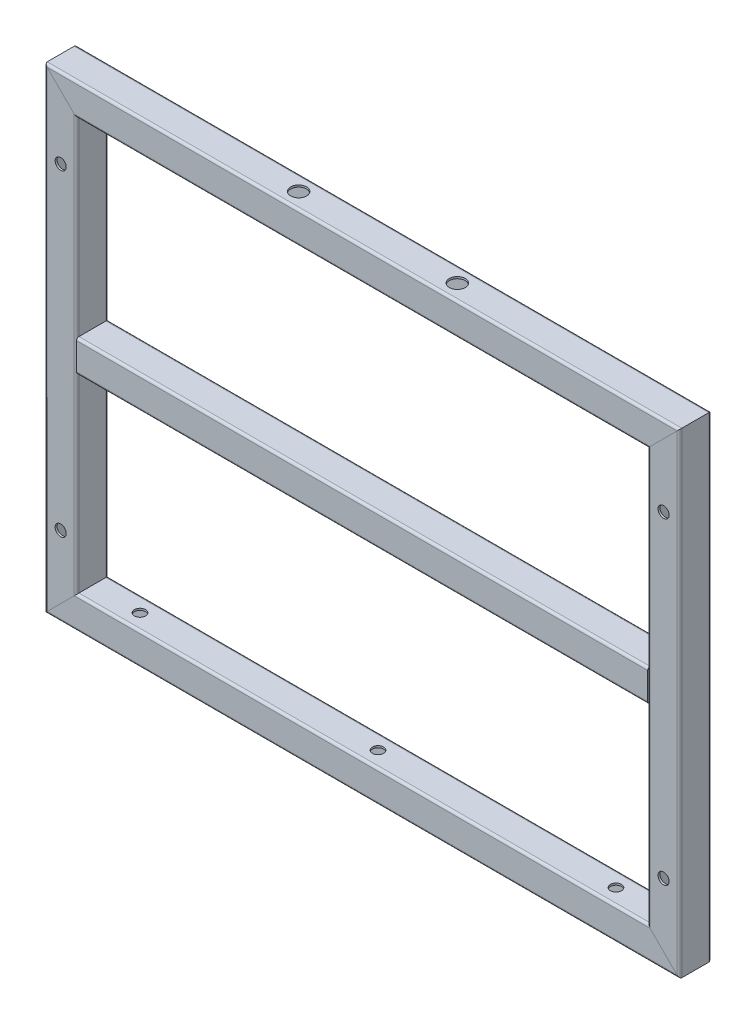
from build123d import *

# Parameters (mm, degrees)
STRUCTURAL_MEMBER1_DEPTH      = 395.142135624
STRUCTURAL_MEMBER1_DEPTH_BACK = 15.142135624
STRUCTURAL_MEMBER1_2_DEPTH    = 310.284271247
STRUCTURAL_MEMBER1_3_DEPTH    = 410.284271247
STRUCTURAL_MEMBER1_4_DEPTH    = 310.284271247
STRUCTURAL_MEMBER1_5_DEPTH    = 382
SKETCH3_R                     = 3.5
CUT_EXTRUDE1_DEPTH            = 251.79872408
SKETCH4_R                     = 5
CUT_EXTRUDE2_DEPTH            = 10
SKETCH5_R                     = 3.5
CUT_EXTRUDE3_DEPTH            = 20


with BuildPart() as part:
    # Sketch1 → Structural Member1 (new, two sides: drawn at the far end of the back side and taken through both)
    with BuildSketch(Plane(origin=(190, 140, 0), x_dir=(0, -1, 0), z_dir=(-1, 0, 0)).offset(-STRUCTURAL_MEMBER1_DEPTH_BACK)):
        with BuildLine():
            Line((-8.5, -10), (8.5, -10))
            ThreePointArc((8.5, -10), (9.560660172, -9.560660172), (10, -8.5))
            Line((10, -8.5), (10, 8.5))
            ThreePointArc((10, 8.5), (9.560660172, 9.560660172), (8.5, 10))
            Line((8.5, 10), (-8.5, 10))
            ThreePointArc((-8.5, 10), (-9.560660172, 9.560660172), (-10, 8.5))
            Line((-10, 8.5), (-10, -8.5))
            ThreePointArc((-10, -8.5), (-9.560660172, -9.560660172), (-8.5, -10))
        make_face()
        with BuildLine():
            Line((-8.5, -8.8), (8.5, -8.8))
            ThreePointArc((8.5, -8.8), (8.712132034, -8.712132034), (8.8, -8.5))
            Line((8.8, -8.5), (8.8, 8.5))
            ThreePointArc((8.8, 8.5), (8.712132034, 8.712132034), (8.5, 8.8))
            Line((8.5, 8.8), (-8.5, 8.8))
            ThreePointArc((-8.5, 8.8), (-8.712132034, 8.712132034), (-8.8, 8.5))
            Line((-8.8, 8.5), (-8.8, -8.5))
            ThreePointArc((-8.8, -8.5), (-8.712132034, -8.712132034), (-8.5, -8.8))
        make_face(mode=Mode.SUBTRACT)
    extrude(amount=STRUCTURAL_MEMBER1_DEPTH + STRUCTURAL_MEMBER1_DEPTH_BACK)

    # Structural Member1 mitre 1
    split(bisect_by=Plane(origin=(190, 140, 0), x_dir=(-0.707106781, -0.707106781, 0), z_dir=(-0.707106781, 0.707106781, 0)), keep=Keep.TOP)

    # Structural Member1 mitre 2
    split(bisect_by=Plane(origin=(-190, 140, 0), x_dir=(-0.707106781, 0.707106781, 0), z_dir=(0.707106781, 0.707106781, 0)), keep=Keep.TOP)

    # Sketch4 → Cut-Extrude2 (cut)
    with BuildSketch(Plane(origin=(0, 150, 0), x_dir=(-1, 0, 0), z_dir=(0, 1, 0))):
        with Locations((50, 0)):
            Circle(SKETCH4_R)
        with Locations((-50, 0)):
            Circle(SKETCH4_R)
    extrude(amount=-CUT_EXTRUDE2_DEPTH, mode=Mode.SUBTRACT)


with BuildPart() as body_2:
    # Sketch1 on segment 2 (carried to segment 2) → Structural Member1 2 (new body)
    with BuildSketch(Plane(origin=(-190, 155.142135624, 0), x_dir=(1, 0, 0), z_dir=(0, -1, 0))):
        with BuildLine():
            Line((-8.5, -10), (8.5, -10))
            ThreePointArc((8.5, -10), (9.560660172, -9.560660172), (10, -8.5))
            Line((10, -8.5), (10, 8.5))
            ThreePointArc((10, 8.5), (9.560660172, 9.560660172), (8.5, 10))
            Line((8.5, 10), (-8.5, 10))
            ThreePointArc((-8.5, 10), (-9.560660172, 9.560660172), (-10, 8.5))
            Line((-10, 8.5), (-10, -8.5))
            ThreePointArc((-10, -8.5), (-9.560660172, -9.560660172), (-8.5, -10))
        make_face()
        with BuildLine():
            Line((-8.5, -8.8), (8.5, -8.8))
            ThreePointArc((8.5, -8.8), (8.712132034, -8.712132034), (8.8, -8.5))
            Line((8.8, -8.5), (8.8, 8.5))
            ThreePointArc((8.8, 8.5), (8.712132034, 8.712132034), (8.5, 8.8))
            Line((8.5, 8.8), (-8.5, 8.8))
            ThreePointArc((-8.5, 8.8), (-8.712132034, 8.712132034), (-8.8, 8.5))
            Line((-8.8, 8.5), (-8.8, -8.5))
            ThreePointArc((-8.8, -8.5), (-8.712132034, -8.712132034), (-8.5, -8.8))
        make_face(mode=Mode.SUBTRACT)
    extrude(amount=STRUCTURAL_MEMBER1_2_DEPTH)

    # Structural Member1 2 mitre 1
    split(bisect_by=Plane(origin=(-190, 140, 0), x_dir=(0.707106781, -0.707106781, 0), z_dir=(-0.707106781, -0.707106781, 0)), keep=Keep.TOP)

    # Structural Member1 2 mitre 2
    split(bisect_by=Plane(origin=(-190, -140, 0), x_dir=(-0.707106781, -0.707106781, 0), z_dir=(-0.707106781, 0.707106781, 0)), keep=Keep.TOP)


with BuildPart() as body_3:
    # Sketch1 on segment 3 (carried to segment 3) → Structural Member1 3 (new body)
    with BuildSketch(Plane(origin=(-205.142135624, -140, 0), x_dir=(0, 1, 0), z_dir=(1, 0, 0))):
        with BuildLine():
            Line((-8.5, -10), (8.5, -10))
            ThreePointArc((8.5, -10), (9.560660172, -9.560660172), (10, -8.5))
            Line((10, -8.5), (10, 8.5))
            ThreePointArc((10, 8.5), (9.560660172, 9.560660172), (8.5, 10))
            Line((8.5, 10), (-8.5, 10))
            ThreePointArc((-8.5, 10), (-9.560660172, 9.560660172), (-10, 8.5))
            Line((-10, 8.5), (-10, -8.5))
            ThreePointArc((-10, -8.5), (-9.560660172, -9.560660172), (-8.5, -10))
        make_face()
        with BuildLine():
            Line((-8.5, -8.8), (8.5, -8.8))
            ThreePointArc((8.5, -8.8), (8.712132034, -8.712132034), (8.8, -8.5))
            Line((8.8, -8.5), (8.8, 8.5))
            ThreePointArc((8.8, 8.5), (8.712132034, 8.712132034), (8.5, 8.8))
            Line((8.5, 8.8), (-8.5, 8.8))
            ThreePointArc((-8.5, 8.8), (-8.712132034, 8.712132034), (-8.8, 8.5))
            Line((-8.8, 8.5), (-8.8, -8.5))
            ThreePointArc((-8.8, -8.5), (-8.712132034, -8.712132034), (-8.5, -8.8))
        make_face(mode=Mode.SUBTRACT)
    extrude(amount=STRUCTURAL_MEMBER1_3_DEPTH)

    # Structural Member1 3 mitre 1
    split(bisect_by=Plane(origin=(190, -140, 0), x_dir=(0.707106781, -0.707106781, 0), z_dir=(-0.707106781, -0.707106781, 0)), keep=Keep.TOP)

    # Structural Member1 3 mitre 2
    split(bisect_by=Plane(origin=(-190, -140, 0), x_dir=(0.707106781, 0.707106781, 0), z_dir=(0.707106781, -0.707106781, 0)), keep=Keep.TOP)

    # Sketch5 → Cut-Extrude3 (cut)
    with BuildSketch(Plane(origin=(0, -130, 0), x_dir=(-1, 0, 0), z_dir=(0, 1, 0))):
        Circle(SKETCH5_R)
        with Locations((-150, 0)):
            Circle(SKETCH5_R)
        with Locations((150, 0)):
            Circle(SKETCH5_R)
    extrude(amount=-CUT_EXTRUDE3_DEPTH, mode=Mode.SUBTRACT)


with BuildPart() as body_4:
    # Sketch1 on segment 4 (carried to segment 4) → Structural Member1 4 (new body)
    with BuildSketch(Plane(origin=(190, -155.142135624, 0), x_dir=(-1, 0, 0), z_dir=(0, 1, 0))):
        with BuildLine():
            Line((-8.5, -10), (8.5, -10))
            ThreePointArc((8.5, -10), (9.560660172, -9.560660172), (10, -8.5))
            Line((10, -8.5), (10, 8.5))
            ThreePointArc((10, 8.5), (9.560660172, 9.560660172), (8.5, 10))
            Line((8.5, 10), (-8.5, 10))
            ThreePointArc((-8.5, 10), (-9.560660172, 9.560660172), (-10, 8.5))
            Line((-10, 8.5), (-10, -8.5))
            ThreePointArc((-10, -8.5), (-9.560660172, -9.560660172), (-8.5, -10))
        make_face()
        with BuildLine():
            Line((-8.5, -8.8), (8.5, -8.8))
            ThreePointArc((8.5, -8.8), (8.712132034, -8.712132034), (8.8, -8.5))
            Line((8.8, -8.5), (8.8, 8.5))
            ThreePointArc((8.8, 8.5), (8.712132034, 8.712132034), (8.5, 8.8))
            Line((8.5, 8.8), (-8.5, 8.8))
            ThreePointArc((-8.5, 8.8), (-8.712132034, 8.712132034), (-8.8, 8.5))
            Line((-8.8, 8.5), (-8.8, -8.5))
            ThreePointArc((-8.8, -8.5), (-8.712132034, -8.712132034), (-8.5, -8.8))
        make_face(mode=Mode.SUBTRACT)
    extrude(amount=STRUCTURAL_MEMBER1_4_DEPTH)

    # Structural Member1 4 mitre 1
    split(bisect_by=Plane(origin=(190, 140, 0), x_dir=(0.707106781, 0.707106781, 0), z_dir=(0.707106781, -0.707106781, 0)), keep=Keep.TOP)

    # Structural Member1 4 mitre 2
    split(bisect_by=Plane(origin=(190, -140, 0), x_dir=(-0.707106781, 0.707106781, 0), z_dir=(0.707106781, 0.707106781, 0)), keep=Keep.TOP)


with BuildPart() as body_5:
    # Sketch1 on segment 5 (carried to segment 5) → Structural Member1 5 (new body)
    with BuildSketch(Plane.YZ.offset(-191)):
        with BuildLine():
            Line((-8.5, -10), (8.5, -10))
            ThreePointArc((8.5, -10), (9.560660172, -9.560660172), (10, -8.5))
            Line((10, -8.5), (10, 8.5))
            ThreePointArc((10, 8.5), (9.560660172, 9.560660172), (8.5, 10))
            Line((8.5, 10), (-8.5, 10))
            ThreePointArc((-8.5, 10), (-9.560660172, 9.560660172), (-10, 8.5))
            Line((-10, 8.5), (-10, -8.5))
            ThreePointArc((-10, -8.5), (-9.560660172, -9.560660172), (-8.5, -10))
        make_face()
        with BuildLine():
            Line((-8.5, -8.8), (8.5, -8.8))
            ThreePointArc((8.5, -8.8), (8.712132034, -8.712132034), (8.8, -8.5))
            Line((8.8, -8.5), (8.8, 8.5))
            ThreePointArc((8.8, 8.5), (8.712132034, 8.712132034), (8.5, 8.8))
            Line((8.5, 8.8), (-8.5, 8.8))
            ThreePointArc((-8.5, 8.8), (-8.712132034, 8.712132034), (-8.8, 8.5))
            Line((-8.8, 8.5), (-8.8, -8.5))
            ThreePointArc((-8.8, -8.5), (-8.712132034, -8.712132034), (-8.5, -8.8))
        make_face(mode=Mode.SUBTRACT)
    extrude(amount=STRUCTURAL_MEMBER1_5_DEPTH)

    # Structural Member1 5 mitre 1
    split(bisect_by=Plane.YZ.offset(-180), keep=Keep.TOP)

    # Structural Member1 5 mitre 2
    split(bisect_by=Plane(origin=(180, 0, 0), x_dir=(0, -1, 0), z_dir=(-1, 0, 0)), keep=Keep.TOP)


with BuildPart() as cut_extrude1_tool:
    # Sketch3 → Cut-Extrude1 (new, through all)
    with BuildSketch(Plane.XY.offset(10)):
        with Locations((-190, 100)):
            Circle(SKETCH3_R)
        with Locations((-190, -100)):
            Circle(SKETCH3_R)
        with Locations((190, -100)):
            Circle(SKETCH3_R)
        with Locations((190, 100)):
            Circle(SKETCH3_R)
    extrude(amount=-CUT_EXTRUDE1_DEPTH)


with BuildPart() as body_2_1:
    add(body_2.part)

    # Cut-Extrude1: cut by cut_extrude1_tool
    add(cut_extrude1_tool.part, mode=Mode.SUBTRACT)


with BuildPart() as body_4_1:
    add(body_4.part)

    # Cut-Extrude1: cut by cut_extrude1_tool
    add(cut_extrude1_tool.part, mode=Mode.SUBTRACT)


solid = Compound([part.part, body_3.part, body_5.part, body_2_1.part, body_4_1.part])
